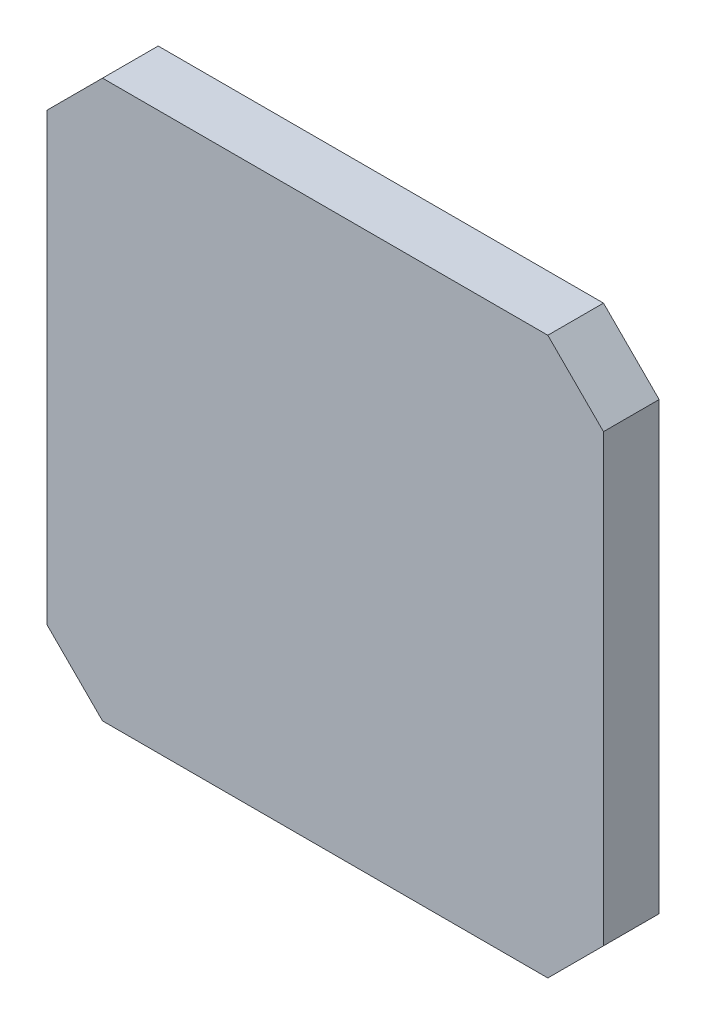
SolidWorks part; units mm, degrees
material "Q235-A"
ref_plane "Front Plane" through (0, 0, 0) normal (0, 0, 1) x (1, 0, 0)
ref_plane "Top Plane" through (0, 0, 0) normal (0, 1, 0) x (1, 0, 0)
ref_plane "Right Plane" through (0, 0, 0) normal (1, 0, 0) x (0, 0, -1)
sketch "Sketch1" plane through (0, 0, 0) normal (0, 0, 1) x (1, 0, 0)
  line L1 (-24.4588, 28.4198) -> (25.5412, 28.4198)
  line L2 (-24.4588, 28.4198) -> (-24.4588, -21.5802)
  line L3 (-24.4588, -21.5802) -> (25.5412, -21.5802)
  line L4 (25.5412, 28.4198) -> (25.5412, -21.5802)
  dimension "D1" = 50
  dimension "D2" = 50
extrude "Boss-Extrude1" add sketch "Sketch1" along normal blind 5
chamfer "Chamfer1" distance 5 angle 45 4 edges at (-24.4588, -21.5802, 2.5) (25.5412, -21.5802, 2.5) (25.5412, 28.4198, 2.5) (-24.4588, 28.4198, 2.5)
